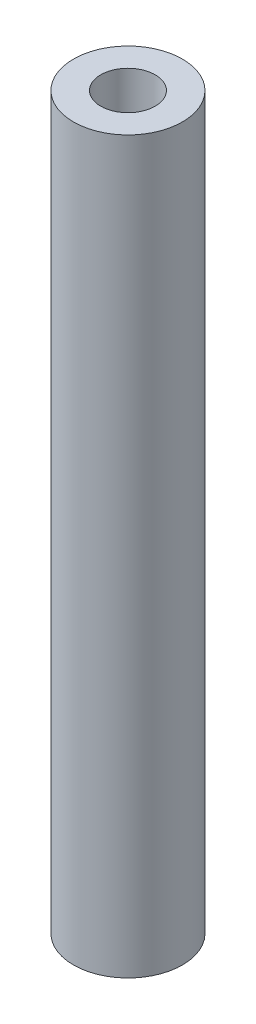
from build123d import *

# Parameters (mm, degrees)
SKETCH1_R           = 1
SKETCH1_R_2         = 0.5
BOSS_EXTRUDE1_DEPTH = 13.4


with BuildPart() as part:
    # Sketch1 → Boss-Extrude1 (new body)
    with BuildSketch(Plane(origin=(0, 0, 0), x_dir=(1, 0, 0), z_dir=(0, 1, 0))):
        with Locations(Location((0, 0, 0), (0, 0, 270))):
            Circle(SKETCH1_R)
        with Locations(Location((0, 0, 0), (0, 0, 270))):
            Circle(SKETCH1_R_2, mode=Mode.SUBTRACT)
    extrude(amount=BOSS_EXTRUDE1_DEPTH)


solid = part.part
